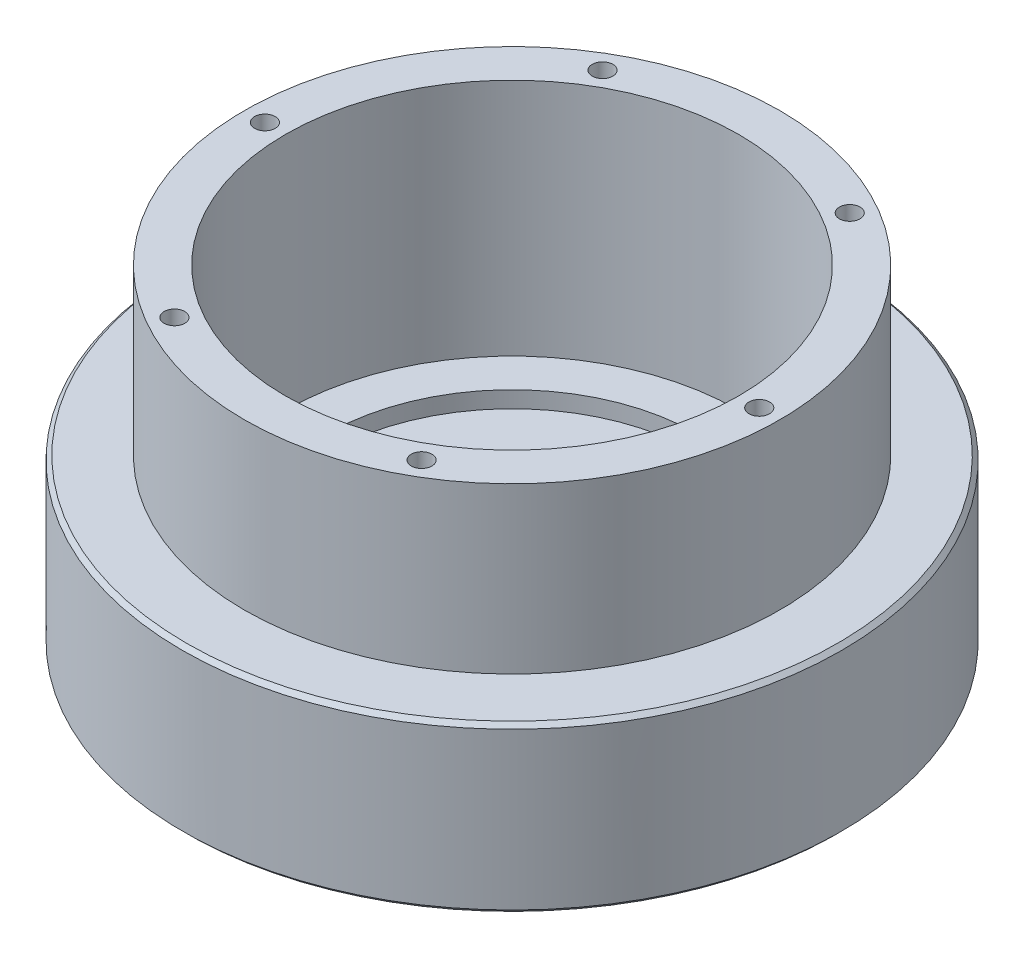
from build123d import *

# Parameters (mm, degrees)
M3_TAPPED_HOLE1_D     = 2.5
M3_TAPPED_HOLE1_DEPTH = 7.5
M3_TAPPED_HOLE1_TIP   = 0.751075774
CHAMFER1_SIZE         = 0.5
M4_TAPPED_HOLE1_D     = 3.3
M4_TAPPED_HOLE1_DEPTH = 10.1
M4_TAPPED_HOLE1_TIP   = 0.991420021
M3_TAPPED_HOLE2_D     = 2.5
M3_TAPPED_HOLE2_DEPTH = 7.5
M3_TAPPED_HOLE2_TIP   = 0.751075774
M3_TAPPED_HOLE3_D     = 2.5
M3_TAPPED_HOLE3_DEPTH = 7.5
M3_TAPPED_HOLE3_TIP   = 0.751075774
M4_TAPPED_HOLE2_D     = 3.3
M4_TAPPED_HOLE2_DEPTH = 10.1
M4_TAPPED_HOLE2_TIP   = 0.991420021


with BuildPart() as part:
    # Sketch1 → Revolve1 (revolve)
    with BuildSketch(Plane.XY, mode=Mode.PRIVATE) as revolve1_sk:
        Polygon((0, 0), (40, 0), (40, 20), (32.5, 20), (32.5, 40), (0, 40), align=None)
    revolve(revolve1_sk.sketch.rotate(Axis((0, 0, 0), (0, 1, 0)), 90), axis=Axis((0, 0, 0), (0, 1, 0)))

    # Sketch2 → Cut-Revolve1 (revolve, cut)
    with BuildSketch(Plane.XY, mode=Mode.PRIVATE) as cut_revolve1_sk:
        Polygon((0, 40), (27.5, 40), (27.5, 11), (22.5, 11), (22.5, 9), (16, 9), (16, 0), (0, 0), align=None)
    revolve(cut_revolve1_sk.sketch.rotate(Axis((0, 0, 0), (0, 1, 0)), 90), axis=Axis((0, 0, 0), (0, 1, 0)), mode=Mode.SUBTRACT)

    # M3 Tapped Hole1
    with Locations(Plane(origin=(0, 40, 0), x_dir=(1, 0, 0), z_dir=(0, 1, 0))):
        with Locations((-30, 0), (-15, 25.980762114), (15, 25.980762114), (30, 0), (15, -25.980762114), (-15, -25.980762114), (0, 0)):
            Hole(M3_TAPPED_HOLE1_D / 2, depth=M3_TAPPED_HOLE1_DEPTH)
            with Locations((0, 0, -(M3_TAPPED_HOLE1_DEPTH + M3_TAPPED_HOLE1_TIP / 2))):  # 118° drill point
                Cone(0, M3_TAPPED_HOLE1_D / 2, M3_TAPPED_HOLE1_TIP, mode=Mode.SUBTRACT)

    # Chamfer1
    chamfer1_edges = [part.edges().sort_by_distance(p)[0] for p in [
        (0, 0, 40),
        (0, 20, 40),
    ]]
    chamfer(chamfer1_edges, length=CHAMFER1_SIZE)

    # M4 Tapped Hole1
    with Locations(Plane(origin=(0, 0, 0), x_dir=(-1, 0, 0), z_dir=(0, -1, 0))):
        with Locations((18.814495684, 29.412337557)):
            Hole(M4_TAPPED_HOLE1_D / 2, depth=M4_TAPPED_HOLE1_DEPTH)
            with Locations((0, 0, -(M4_TAPPED_HOLE1_DEPTH + M4_TAPPED_HOLE1_TIP / 2))):  # 118° drill point
                Cone(0, M4_TAPPED_HOLE1_D / 2, M4_TAPPED_HOLE1_TIP, mode=Mode.SUBTRACT)

    # M3 Tapped Hole2
    with Locations(Plane(origin=(0, 0, 0), x_dir=(-1, 0, 0), z_dir=(0, -1, 0))):
        with Locations((-34.334850717, 15.469705912), (-25.834850717, 0.747274048)):
            Hole(M3_TAPPED_HOLE2_D / 2, depth=M3_TAPPED_HOLE2_DEPTH)
            with Locations((0, 0, -(M3_TAPPED_HOLE2_DEPTH + M3_TAPPED_HOLE2_TIP / 2))):  # 118° drill point
                Cone(0, M3_TAPPED_HOLE2_D / 2, M3_TAPPED_HOLE2_TIP, mode=Mode.SUBTRACT)

    # M3 Tapped Hole3
    with Locations(Plane(origin=(0, 0, 0), x_dir=(-1, 0, 0), z_dir=(0, -1, 0))):
        with Locations((4.989178136, 28.35848998), (-12.331329939, 18.35848998), (-29.651838015, 8.35848998)):
            Hole(M3_TAPPED_HOLE3_D / 2, depth=M3_TAPPED_HOLE3_DEPTH)
            with Locations((0, 0, -(M3_TAPPED_HOLE3_DEPTH + M3_TAPPED_HOLE3_TIP / 2))):  # 118° drill point
                Cone(0, M3_TAPPED_HOLE3_D / 2, M3_TAPPED_HOLE3_TIP, mode=Mode.SUBTRACT)

    # M4 Tapped Hole2
    with Locations(Plane(origin=(0, 0, 0), x_dir=(-1, 0, 0), z_dir=(0, -1, 0))):
        with Locations((22.910254038, -19.681724008), (5.589745962, -29.681724008)):
            Hole(M4_TAPPED_HOLE2_D / 2, depth=M4_TAPPED_HOLE2_DEPTH)
            with Locations((0, 0, -(M4_TAPPED_HOLE2_DEPTH + M4_TAPPED_HOLE2_TIP / 2))):  # 118° drill point
                Cone(0, M4_TAPPED_HOLE2_D / 2, M4_TAPPED_HOLE2_TIP, mode=Mode.SUBTRACT)


solid = part.part
